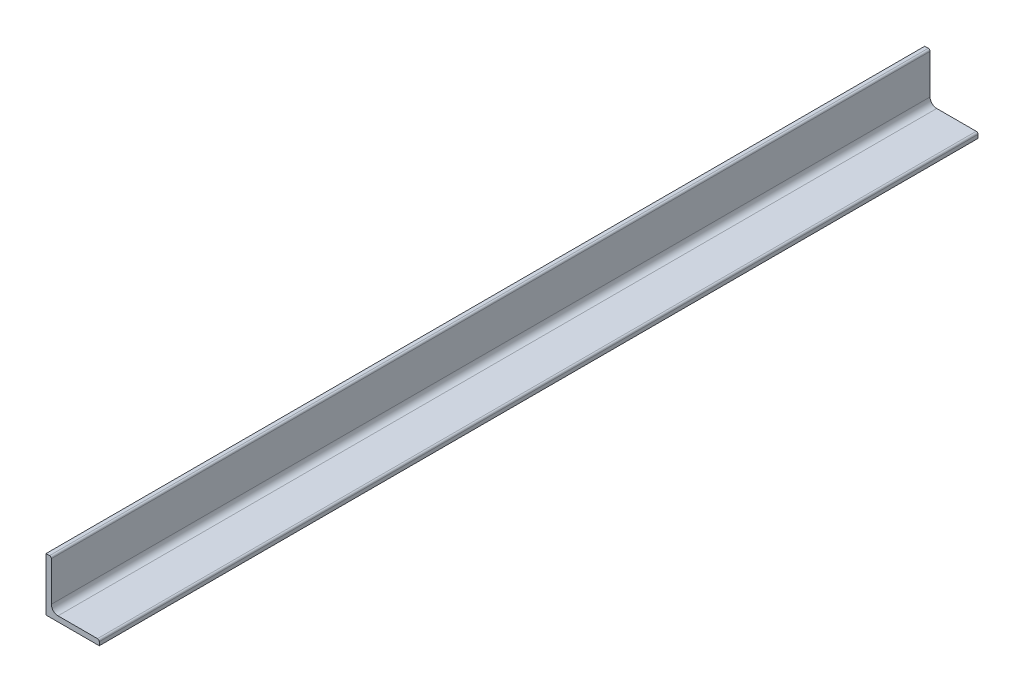
SolidWorks part; units mm, degrees
material "Q235B"
ref_plane "Plane1" through (0, 0, 0) normal (0, 0, 1) x (1, 0, 0)
ref_plane "Plane2" through (0, 0, 0) normal (0, 1, 0) x (1, 0, 0)
ref_plane "Plane3" through (0, 0, 0) normal (1, 0, 0) x (0, 0, -1)
sketch "Sketch1" plane through (0, 0, 0) normal (0, 0, 1) x (1, 0, 0)
  line L0 (0, 0) -> (0, 40)
  line L1 (0, 20) -> (4, 20) construction
  line L2 (4, 38.6667) -> (4, 9)
  line L3 (9, 4) -> (38.6667, 4)
  line L4 (20, 4) -> (20, 0) construction
  line L5 (40, 0) -> (0, 0)
  line L6 (0, 40) -> (2.6667, 40)
  line L7 (40, 0) -> (40, 2.6667)
  arc A0 (40, 2.6667) -> (38.6667, 4) centre (38.6667, 2.6667) ccw
  arc A1 (2.6667, 40) -> (4, 38.6667) centre (2.6667, 38.6667) cw
  arc A2 (9, 4) -> (4, 9) centre (9, 9) cw
  point P10 (20, 0)
  point P14 (0, 20)
  point P15 (4, 20)
  point P16 (20, 4)
  point P17 (4, 40)
  point P18 (40, 4)
  point P21 (40, 4)
  point P24 (4, 40)
extrude "Boss-Extrude1" add sketch "Sketch1" along normal blind 660 contours L3 A0 L7 L5 L0 L6 A1 L2 A2
equation "\"D2@Sketch1\" = \"D1@Sketch1\" / 3"
